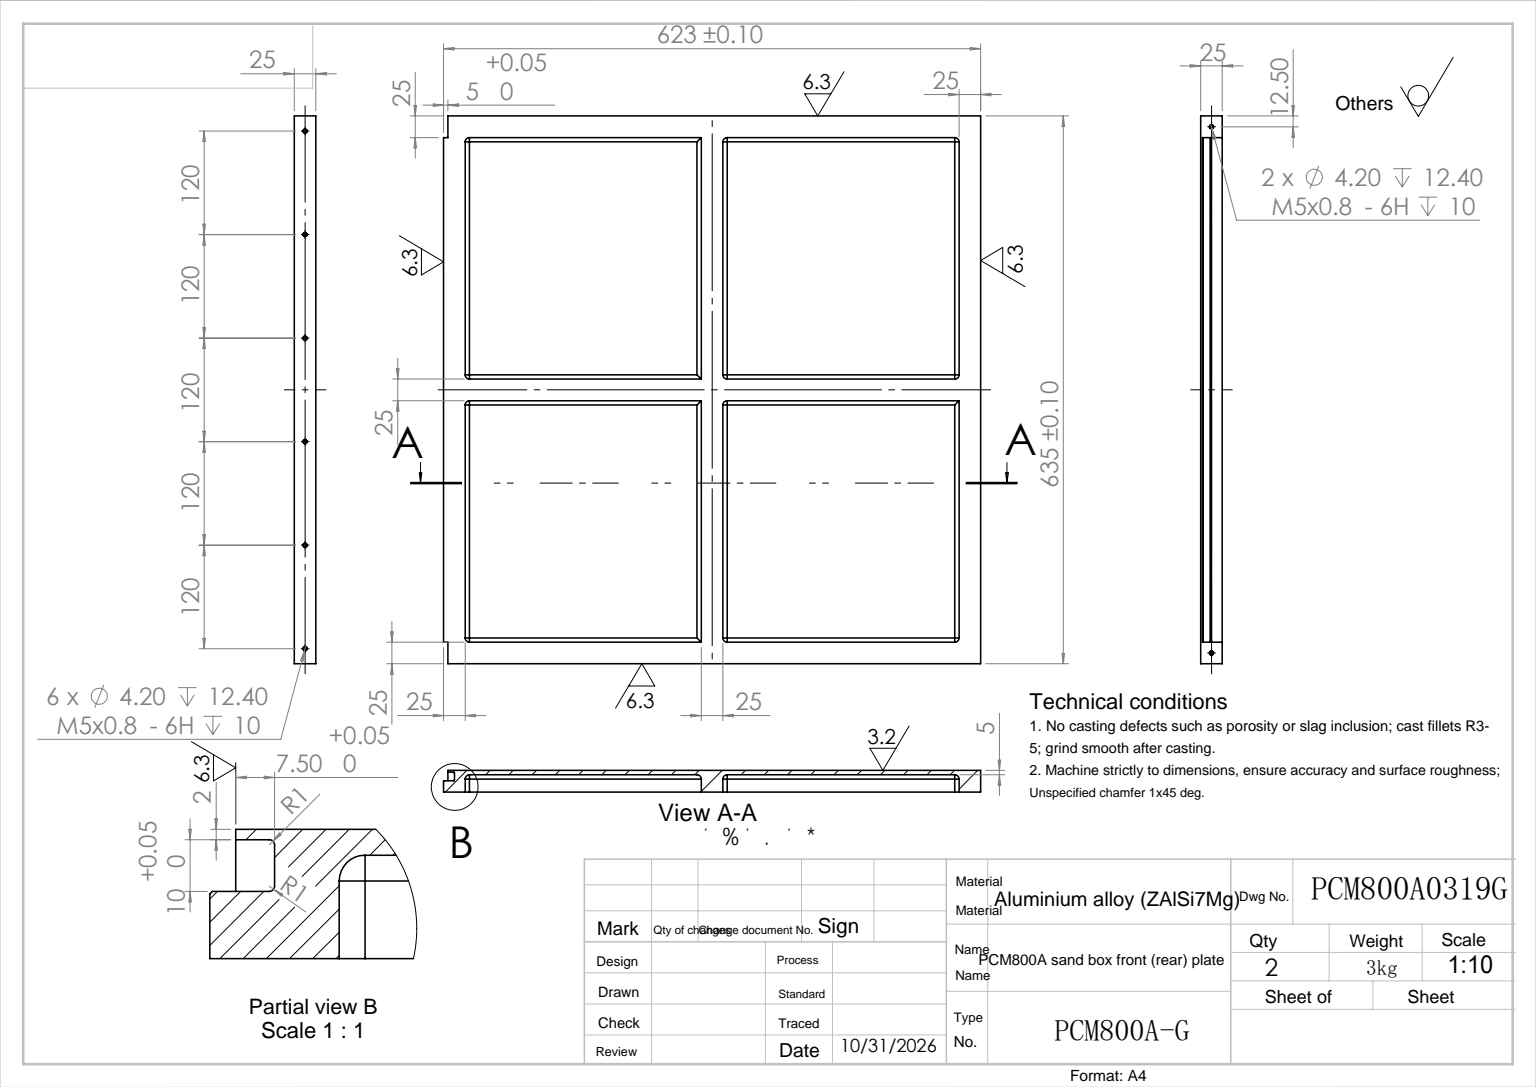
from build123d import *

# Parameters (mm, degrees)
SKETCH_1_W           = 623
SKETCH_1_H           = 635
EXTRUDE_1_DEPTH      = 5
SKETCH_2_W           = 25
SKETCH_2_H           = 635
EXTRUDE_2_DEPTH      = 20
SKETCH_3_W           = 25
SKETCH_3_H           = 635
EXTRUDE_3_DEPTH      = 20
CUT_EXTRUDE_1_DEPTH  = 890.932019876
CHAMFER_1_SIZE       = 0.5
SKETCH_7_W           = 573
SKETCH_7_H           = 25
EXTRUDE_4_DEPTH      = 20
SKETCH_8_W           = 573
SKETCH_8_H           = 25
EXTRUDE_5_DEPTH      = 20
SKETCH_9_W           = 573
SKETCH_9_H           = 25
EXTRUDE_6_DEPTH      = 20
SKETCH_10_W          = 25
SKETCH_10_H          = 585
EXTRUDE_7_DEPTH      = 20
EXTRUDE_8_DEPTH      = 25
CUT_EXTRUDE_2_DEPTH  = 25
EXTRUDE_START        = -25
EXTRUDE_9_DEPTH      = 25
CUT_EXTRUDE_3_DEPTH  = 25
M5X0_8_1_D           = 4.2
M5X0_8_1_DEPTH       = 12.4
M5X0_8_1_CBORE_D     = 5
M5X0_8_1_CBORE_DEPTH = 10
M5X0_8_1_TIP         = 1.2618073
M5X0_8_2_D           = 4.2
M5X0_8_2_DEPTH       = 12.4
M5X0_8_2_CBORE_D     = 5
M5X0_8_2_CBORE_DEPTH = 10
M5X0_8_2_TIP         = 1.2618073
FILLET_1_R           = 5


with BuildPart() as part:
    # 草图1 → 拉伸1 (new body)
    with BuildSketch(Plane.XY):
        with Locations((311.5, 317.5)):
            Rectangle(SKETCH_1_W, SKETCH_1_H)
    extrude(amount=EXTRUDE_1_DEPTH)

    # 草图2 → 拉伸2 (add)
    with BuildSketch(Plane.XY.offset(5)):
        with Locations((12.5, 317.5)):
            Rectangle(SKETCH_2_W, SKETCH_2_H)
    extrude(amount=EXTRUDE_2_DEPTH)

    # 草图3 → 拉伸3 (add)
    with BuildSketch(Plane.XY.offset(5)):
        with Locations((610.5, 317.5)):
            Rectangle(SKETCH_3_W, SKETCH_3_H)
    extrude(amount=EXTRUDE_3_DEPTH)

    # 草图4 → 切除-拉伸1 (cut, through all)
    with BuildSketch(Plane(origin=(0, 635, 0), x_dir=(-1, 0, 0), z_dir=(0, 1, 0))):
        with BuildLine():
            Line((0, 0), (-5, 0))
            Line((-5, 0), (-5, 2))
            Line((-5, 2), (-11.5, 2))
            ThreePointArc((-11.5, 2), (-12.207106781, 2.292893219), (-12.5, 3))
            Line((-12.5, 3), (-12.5, 11))
            ThreePointArc((-12.5, 11), (-12.207106781, 11.707106781), (-11.5, 12))
            Line((-11.5, 12), (0, 12))
            Line((0, 12), (0, 0))
        make_face()
    extrude(amount=-CUT_EXTRUDE_1_DEPTH, mode=Mode.SUBTRACT)

    # 倒角1
    chamfer_1_edges = [part.edges().sort_by_distance(p)[0] for p in [
        (0, 317.5, 12),
    ]]
    chamfer(chamfer_1_edges, length=CHAMFER_1_SIZE)

    # 草图7 → 拉伸4 (add)
    with BuildSketch(Plane.XY.offset(5)):
        with Locations((311.5, 622.5)):
            Rectangle(SKETCH_7_W, SKETCH_7_H)
    extrude(amount=EXTRUDE_4_DEPTH)

    # 草图8 → 拉伸5 (add)
    with BuildSketch(Plane.XY.offset(5)):
        with Locations((311.5, 12.5)):
            Rectangle(SKETCH_8_W, SKETCH_8_H)
    extrude(amount=EXTRUDE_5_DEPTH)

    # 草图9 → 拉伸6 (add)
    with BuildSketch(Plane.XY.offset(5)):
        with Locations((311.5, 317.5)):
            Rectangle(SKETCH_9_W, SKETCH_9_H)
    extrude(amount=EXTRUDE_6_DEPTH)

    # 草图10 → 拉伸7 (add)
    with BuildSketch(Plane.XY.offset(5)):
        with Locations((311.5, 317.5)):
            Rectangle(SKETCH_10_W, SKETCH_10_H)
    extrude(amount=EXTRUDE_7_DEPTH)

    # 草图11 → 拉伸8 (add)
    with BuildSketch(Plane(origin=(0, 635, 0), x_dir=(-1, 0, 0), z_dir=(0, 1, 0))):
        with BuildLine():
            Line((-5, 2), (-5, 12))
            Line((-5, 12), (-11.5, 12))
            ThreePointArc((-11.5, 12), (-12.207106781, 11.707106781), (-12.5, 11))
            Line((-12.5, 11), (-12.5, 3))
            ThreePointArc((-12.5, 3), (-12.207106781, 2.292893219), (-11.5, 2))
            Line((-11.5, 2), (-5, 2))
        make_face()
    extrude(amount=-EXTRUDE_8_DEPTH)

    # 草图12 → 切除-拉伸2 (cut)
    with BuildSketch(Plane(origin=(0, 635, 0), x_dir=(-1, 0, 0), z_dir=(0, 1, 0))):
        Polygon((-5, 12), (-0.5, 12), (0, 12.5), (0, 25), (-5, 25), align=None)
    extrude(amount=-CUT_EXTRUDE_2_DEPTH, mode=Mode.SUBTRACT)

    # 草图13 → 拉伸9 (add)
    with BuildSketch(Plane.XZ.offset(EXTRUDE_START)):
        with BuildLine():
            Line((5, 2), (5, 12))
            Line((5, 12), (11.5, 12))
            ThreePointArc((11.5, 12), (12.207106781, 11.707106781), (12.5, 11))
            Line((12.5, 11), (12.5, 3))
            ThreePointArc((12.5, 3), (12.207106781, 2.292893219), (11.5, 2))
            Line((11.5, 2), (5, 2))
        make_face()
    extrude(amount=EXTRUDE_9_DEPTH)

    # 草图14 → 切除-拉伸3 (cut)
    with BuildSketch(Plane.XZ):
        Polygon((5, 12), (5, 25), (0, 25), (0, 12.5), (0.5, 12), align=None)
    extrude(amount=-CUT_EXTRUDE_3_DEPTH, mode=Mode.SUBTRACT)

    # M5x0.8 螺纹孔1
    with Locations(Plane(origin=(623, 617.5, 12.5), x_dir=(0, 0, 1), z_dir=(1, 0, 0))):
        with Locations((0, 0), (0, 120), (0, 240), (0, 360), (0, 480), (0, 600)):
            CounterBoreHole(M5X0_8_1_D / 2, M5X0_8_1_CBORE_D / 2, M5X0_8_1_CBORE_DEPTH, depth=M5X0_8_1_DEPTH)
            with Locations((0, 0, -(M5X0_8_1_DEPTH + M5X0_8_1_TIP / 2))):  # 118° drill point
                Cone(0, M5X0_8_1_D / 2, M5X0_8_1_TIP, mode=Mode.SUBTRACT)

    # M5x0.8 螺纹孔2
    with Locations(Plane(origin=(5, 12.5, 12.5), x_dir=(0, 0, -1), z_dir=(-1, 0, 0))):
        with Locations((0, 0), (0, -610)):
            CounterBoreHole(M5X0_8_2_D / 2, M5X0_8_2_CBORE_D / 2, M5X0_8_2_CBORE_DEPTH, depth=M5X0_8_2_DEPTH)
            with Locations((0, 0, -(M5X0_8_2_DEPTH + M5X0_8_2_TIP / 2))):  # 118° drill point
                Cone(0, M5X0_8_2_D / 2, M5X0_8_2_TIP, mode=Mode.SUBTRACT)

    # 圆角1
    fillet_1_edges = [part.edges().sort_by_distance(p)[0] for p in [
        (461, 25, 5),
        (598, 25, 15),
        (598, 165, 5),
        (25, 470, 5),
        (25, 330, 15),
        (162, 305, 5),
        (25, 305, 15),
        (461, 330, 5),
        (598, 330, 15),
        (162, 330, 5),
        (324, 330, 15),
        (461, 305, 5),
        (162, 25, 5),
        (461, 610, 5),
        (299, 165, 5),
        (299, 470, 5),
        (324, 165, 5),
        (324, 305, 15),
        (324, 25, 15),
        (324, 470, 5),
        (324, 610, 15),
        (598, 470, 5),
        (162, 610, 5),
        (25, 610, 15),
        (598, 610, 15),
        (25, 165, 5),
        (25, 25, 15),
    ]]
    fillet(fillet_1_edges, radius=FILLET_1_R)


solid = part.part
